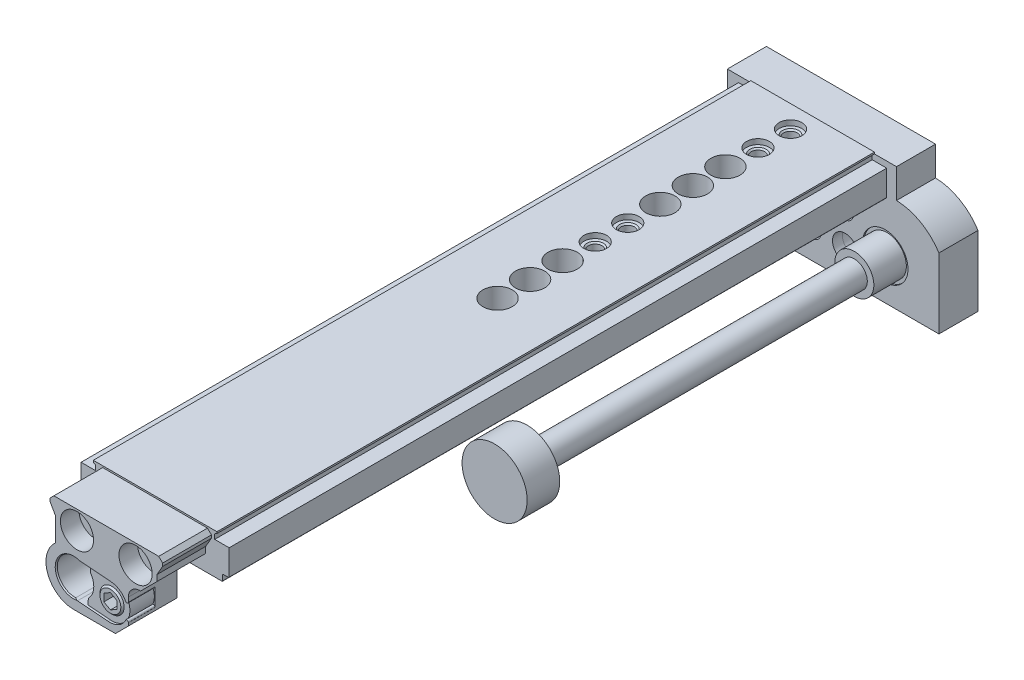
from build123d import *

# Parameters (mm, degrees)
BOSS_EXTRUDE1_DEPTH = 12
CUT_EXTRUDE1_DEPTH  = 3.5
CUT_EXTRUDE2_DEPTH  = 3.5
CUT_EXTRUDE3_DEPTH  = 2.5
SKETCH15_W          = 7
SKETCH15_H          = 0.5
BOSS_EXTRUDE2_DEPTH = 202
BOSS_EXTRUDE3_DEPTH = 15
SKETCH19_R          = 5.1
CUT_EXTRUDE4_DEPTH  = 5.7
SKETCH20_R          = 5.1
CUT_EXTRUDE5_DEPTH  = 5.7
SKETCH21_R          = 2.75
CUT_EXTRUDE6_DEPTH  = 20.6
SKETCH22_R          = 2.75
CUT_EXTRUDE7_DEPTH  = 20.6
SKETCH25_W          = 4.5
SKETCH25_H          = 12.4
SKETCH26_W          = 4.5
SKETCH26_H          = 12.4
SKETCH27_W          = 4.5
SKETCH27_H          = 12.4
SKETCH30_W          = 4.5
SKETCH30_H          = 12.4
SKETCH31_W          = 4.5
SKETCH31_H          = 12.4
SKETCH32_W          = 4.5
SKETCH32_H          = 12.4
CUT_EXTRUDE8_DEPTH  = 8.2
BOSS_EXTRUDE4_START = 7.5
BOSS_EXTRUDE4_DEPTH = 7.5
CUT_EXTRUDE9_DEPTH  = 5.2


with BuildPart() as part:
    # Sketch1 → Boss-Extrude1 (new body)
    with BuildSketch(Plane.XY):
        with BuildLine():
            Line((0, 38), (0, 0))
            Line((0, 0), (65, 0))
            Line((65, 0), (65, 21.556260866))
            ThreePointArc((65, 21.556260866), (59.406255266, 26.898722152), (51.96, 28.992798379))
            Line((51.96, 28.992798379), (51.96, 38))
            Line((51.96, 38), (0, 38))
        make_face()
    extrude(amount=BOSS_EXTRUDE1_DEPTH)

    # Sketch2 → Cut-Revolve1 (revolve, cut)
    with BuildSketch(Plane(origin=(0, 8.5, 0), x_dir=(1, 0, 0), z_dir=(0, 1, 0)), mode=Mode.PRIVATE) as cut_revolve1_sk:
        Polygon((16.2, 0), (20.2, 0), (20.2, -9), (20.1, -9), (20.1, -12), (16.2, -12), align=None)
    revolve(cut_revolve1_sk.sketch.rotate(Axis((16.2, 8.5, 12), (0, 0, -1)), 180), axis=Axis((16.2, 8.5, 12), (0, 0, -1)), mode=Mode.SUBTRACT)

    # Sketch3 → Cut-Revolve2 (revolve, cut)
    with BuildSketch(Plane(origin=(0, 8.5, 0), x_dir=(1, 0, 0), z_dir=(0, 1, 0)), mode=Mode.PRIVATE) as cut_revolve2_sk:
        Polygon((36.2, 0), (40.2, 0), (40.2, -9), (40.1, -9), (40.1, -12), (36.2, -12), align=None)
    revolve(cut_revolve2_sk.sketch.rotate(Axis((36.2, 8.5, 12), (0, 0, -1)), 180), axis=Axis((36.2, 8.5, 12), (0, 0, -1)), mode=Mode.SUBTRACT)

    # Sketch4 → Cut-Revolve3 (revolve, cut)
    with BuildSketch(Plane(origin=(0, 8.5, 0), x_dir=(1, 0, 0), z_dir=(0, 1, 0)), mode=Mode.PRIVATE) as cut_revolve3_sk:
        Polygon((26.2, 0), (29.7, 0), (29.7, -1.6), (28.7, -1.6), (28.267, -1.849992667), (28.267, -11.750007333), (28.7, -12), (26.2, -12), align=None)
    revolve(cut_revolve3_sk.sketch.rotate(Axis((26.2, 8.5, 12), (0, 0, -1)), 180), axis=Axis((26.2, 8.5, 12), (0, 0, -1)), mode=Mode.SUBTRACT)

    # Sketch5 → Cut-Revolve4 (revolve, cut)
    with BuildSketch(Plane(origin=(0, 18.5, 0), x_dir=(1, 0, 0), z_dir=(0, 1, 0)), mode=Mode.PRIVATE) as cut_revolve4_sk:
        Polygon((16.2, 0), (19.7, 0), (19.7, -1.6), (18.7, -1.6), (18.267, -1.849992667), (18.267, -11.750007333), (18.7, -12), (16.2, -12), align=None)
    revolve(cut_revolve4_sk.sketch.rotate(Axis((16.2, 18.5, 12), (0, 0, -1)), 180), axis=Axis((16.2, 18.5, 12), (0, 0, -1)), mode=Mode.SUBTRACT)

    # Sketch6 → Cut-Revolve5 (revolve, cut)
    with BuildSketch(Plane(origin=(0, 18.5, 0), x_dir=(1, 0, 0), z_dir=(0, 1, 0)), mode=Mode.PRIVATE) as cut_revolve5_sk:
        Polygon((26.2, 0), (29.7, 0), (29.7, -1.6), (28.7, -1.6), (28.267, -1.849992667), (28.267, -11.750007333), (28.7, -12), (26.2, -12), align=None)
    revolve(cut_revolve5_sk.sketch.rotate(Axis((26.2, 18.5, 12), (0, 0, -1)), 180), axis=Axis((26.2, 18.5, 12), (0, 0, -1)), mode=Mode.SUBTRACT)

    # Sketch7 → Cut-Revolve6 (revolve, cut)
    with BuildSketch(Plane(origin=(0, 18.5, 0), x_dir=(1, 0, 0), z_dir=(0, 1, 0)), mode=Mode.PRIVATE) as cut_revolve6_sk:
        Polygon((36.2, 0), (39.7, 0), (39.7, -1.6), (38.7, -1.6), (38.267, -1.849992667), (38.267, -11.750007333), (38.7, -12), (36.2, -12), align=None)
    revolve(cut_revolve6_sk.sketch.rotate(Axis((36.2, 18.5, 12), (0, 0, -1)), 180), axis=Axis((36.2, 18.5, 12), (0, 0, -1)), mode=Mode.SUBTRACT)

    # Sketch8 → Cut-Revolve7 (revolve, cut)
    with BuildSketch(Plane(origin=(0, 28.5, 0), x_dir=(1, 0, 0), z_dir=(0, 1, 0)), mode=Mode.PRIVATE) as cut_revolve7_sk:
        Polygon((26.2, 0), (29.7, 0), (29.7, -1.6), (28.7, -1.6), (28.267, -1.849992667), (28.267, -11.750007333), (28.7, -12), (26.2, -12), align=None)
    revolve(cut_revolve7_sk.sketch.rotate(Axis((26.2, 28.5, 12), (0, 0, -1)), 180), axis=Axis((26.2, 28.5, 12), (0, 0, -1)), mode=Mode.SUBTRACT)

    # Sketch9 → Cut-Revolve8 (revolve, cut)
    with BuildSketch(Plane(origin=(0, 32.3, 0), x_dir=(1, 0, 0), z_dir=(0, 1, 0)), mode=Mode.PRIVATE) as cut_revolve8_sk:
        with BuildLine():
            Line((17.2, 0), (22.2, 0))
            Line((22.2, 0), (22.2, -5.7))
            Line((22.2, -5.7), (21.95, -5.7))
            Line((21.95, -5.7), (21.95, -1.1))
            ThreePointArc((21.95, -1.1), (21.832842712, -0.817157288), (21.55, -0.7))
            Line((21.55, -0.7), (19.51, -0.7))
            Line((19.51, -0.7), (17.2, -1.540771241))
            Line((17.2, -1.540771241), (17.2, 0))
        make_face()
    revolve(cut_revolve8_sk.sketch.rotate(Axis((17.2, 32.3, 5.7), (0, 0, -1)), 180), axis=Axis((17.2, 32.3, 5.7), (0, 0, -1)), mode=Mode.SUBTRACT)

    # Sketch10 → Cut-Revolve9 (revolve, cut)
    with BuildSketch(Plane(origin=(0, 32.3, 0), x_dir=(1, 0, 0), z_dir=(0, 1, 0)), mode=Mode.PRIVATE) as cut_revolve9_sk:
        with BuildLine():
            Line((35.2, 0), (40.2, 0))
            Line((40.2, 0), (40.2, -5.7))
            Line((40.2, -5.7), (39.95, -5.7))
            Line((39.95, -5.7), (39.95, -1.1))
            ThreePointArc((39.95, -1.1), (39.832842712, -0.817157288), (39.55, -0.7))
            Line((39.55, -0.7), (37.51, -0.7))
            Line((37.51, -0.7), (35.2, -1.540771241))
            Line((35.2, -1.540771241), (35.2, 0))
        make_face()
    revolve(cut_revolve9_sk.sketch.rotate(Axis((35.2, 32.3, 5.7), (0, 0, -1)), 180), axis=Axis((35.2, 32.3, 5.7), (0, 0, -1)), mode=Mode.SUBTRACT)

    # Sketch11 → Cut-Extrude1 (cut)
    with BuildSketch(Plane(origin=(0, 0, 0.7), x_dir=(-1, 0, 0), z_dir=(0, 0, -1))):
        Polygon((-33.2, 33.454700538), (-35.2, 34.609401077), (-37.2, 33.454700538), (-37.2, 31.145299462), (-35.2, 29.990598923), (-33.2, 31.145299462), align=None)
    extrude(amount=-CUT_EXTRUDE1_DEPTH, mode=Mode.SUBTRACT)

    # Sketch12 → Cut-Extrude2 (cut)
    with BuildSketch(Plane(origin=(0, 0, 0.7), x_dir=(-1, 0, 0), z_dir=(0, 0, -1))):
        Polygon((-15.2, 33.454700538), (-17.2, 34.609401077), (-19.2, 33.454700538), (-19.2, 31.145299462), (-17.2, 29.990598923), (-15.2, 31.145299462), align=None)
    extrude(amount=-CUT_EXTRUDE2_DEPTH, mode=Mode.SUBTRACT)

    # Sketch13 → Cut-Revolve10 (revolve, cut)
    with BuildSketch(Plane(origin=(0, 12.5, 0), x_dir=(1, 0, 0), z_dir=(0, 1, 0)), mode=Mode.PRIVATE) as cut_revolve10_sk:
        with BuildLine():
            Line((48.5, 0), (53.5, 0))
            Line((53.5, 0), (53.5, -5.7))
            Line((53.5, -5.7), (52.75, -5.7))
            Line((52.75, -5.7), (52.75, -1.1))
            ThreePointArc((52.75, -1.1), (52.632842712, -0.817157288), (52.35, -0.7))
            Line((52.35, -0.7), (50.81, -0.7))
            Line((50.81, -0.7), (48.5, -1.540771241))
            Line((48.5, -1.540771241), (48.5, 0))
        make_face()
    revolve(cut_revolve10_sk.sketch.rotate(Axis((48.5, 12.5, 5.7), (0, 0, -1)), 180), axis=Axis((48.5, 12.5, 5.7), (0, 0, -1)), mode=Mode.SUBTRACT)

    # Sketch14 → Cut-Extrude3 (cut)
    with BuildSketch(Plane(origin=(0, 0, 0.7), x_dir=(-1, 0, 0), z_dir=(0, 0, -1))):
        Polygon((-46.5, 13.654700538), (-48.5, 14.809401077), (-50.5, 13.654700538), (-50.5, 11.345299462), (-48.5, 10.190598923), (-46.5, 11.345299462), align=None)
    extrude(amount=-CUT_EXTRUDE3_DEPTH, mode=Mode.SUBTRACT)

    # Sketch15 → Cut-Revolve11 (revolve, cut)
    with BuildSketch(Plane(origin=(0, 12.5, 0), x_dir=(1, 0, 0), z_dir=(0, 1, 0)), mode=Mode.PRIVATE) as cut_revolve11_sk:
        with Locations((52, -11.75)):
            Rectangle(SKETCH15_W, SKETCH15_H)
    revolve(cut_revolve11_sk.sketch.rotate(Axis((48.5, 12.5, 12), (0, 0, -1)), 180), axis=Axis((48.5, 12.5, 12), (0, 0, -1)), mode=Mode.SUBTRACT)

    # Sketch16 → Revolve1 (revolve)
    with BuildSketch(Plane(origin=(0, 12.5, 0), x_dir=(1, 0, 0), z_dir=(0, 1, 0)), mode=Mode.PRIVATE) as revolve1_sk:
        Polygon((48.5, -11.5), (54.5, -11.5), (54.5, -21.5), (52.5, -21.5), (52.5, -122), (58.5, -122), (58.5, -132), (48.5, -132), align=None)
    revolve(revolve1_sk.sketch.rotate(Axis((48.5, 12.5, 132), (0, 0, -1)), 180), axis=Axis((48.5, 12.5, 132), (0, 0, -1)))

    # Sketch17 → Boss-Extrude2 (add)
    with BuildSketch(Plane.XY.offset(12)):
        with BuildLine():
            Line((3.45, 36.1), (3.45, 28.05))
            ThreePointArc((3.45, 28.05), (3.508578644, 27.908578644), (3.65, 27.85))
            Line((3.65, 27.85), (5.25, 27.85))
            ThreePointArc((5.25, 27.85), (5.391421356, 27.791421356), (5.45, 27.65))
            Line((5.45, 27.65), (5.45, 26.3))
            ThreePointArc((5.45, 26.3), (5.508578644, 26.158578644), (5.65, 26.1))
            Line((5.65, 26.1), (46.75, 26.1))
            ThreePointArc((46.75, 26.1), (46.891421356, 26.158578644), (46.95, 26.3))
            Line((46.95, 26.3), (46.95, 27.9))
            ThreePointArc((46.95, 27.9), (47.008578644, 28.041421356), (47.15, 28.1))
            Line((47.15, 28.1), (48.75, 28.1))
            ThreePointArc((48.75, 28.1), (48.891421356, 28.158578644), (48.95, 28.3))
            Line((48.95, 28.3), (48.95, 36.1))
            Line((48.95, 36.1), (44.5, 36.1))
            Line((44.5, 36.1), (44.5, 37.595854812))
            Line((44.5, 37.595854812), (45.2, 38))
            Line((45.2, 38), (45.2, 38.5))
            Line((45.2, 38.5), (7.2, 38.5))
            Line((7.2, 38.5), (7.2, 38))
            Line((7.2, 38), (7.9, 37.595854812))
            Line((7.9, 37.595854812), (7.9, 36.1))
            Line((7.9, 36.1), (3.45, 36.1))
        make_face()
    extrude(amount=BOSS_EXTRUDE2_DEPTH)

    # Sketch18 → Boss-Extrude3 (add)
    with BuildSketch(Plane.XY.offset(214)):
        with BuildLine():
            Line((16.18, 10.8), (29, 10.8))
            Line((29, 10.8), (33, 14.8))
            Line((33, 14.8), (33, 22.5))
            ThreePointArc((33, 22.5), (34.025126266, 24.974873734), (36.5, 26))
            Line((36.5, 26), (36.75, 26))
            Line((36.75, 26), (41.75, 31))
            Line((41.75, 31), (41.75, 32.868911087))
            Line((41.75, 32.868911087), (43.5, 35.9))
            Line((43.5, 35.9), (43.5, 36.8))
            Line((43.5, 36.8), (42.3, 38))
            Line((42.3, 38), (10.1, 38))
            Line((10.1, 38), (8.9, 36.8))
            Line((8.9, 36.8), (8.9, 35.9))
            Line((8.9, 35.9), (10.65, 32.868911087))
            Line((10.65, 32.868911087), (10.65, 25.755160726))
            ThreePointArc((10.65, 25.755160726), (8.207582983, 16.352023251), (16.18, 10.8))
        make_face()
    extrude(amount=BOSS_EXTRUDE3_DEPTH)

    # Sketch19 → Cut-Extrude4 (cut)
    with BuildSketch(Plane.XY.offset(229)):
        with Locations((17.2, 32.3)):
            Circle(SKETCH19_R)
    extrude(amount=-CUT_EXTRUDE4_DEPTH, mode=Mode.SUBTRACT)

    # Sketch20 → Cut-Extrude5 (cut)
    with BuildSketch(Plane.XY.offset(229)):
        with Locations((35.2, 32.3)):
            Circle(SKETCH20_R)
    extrude(amount=-CUT_EXTRUDE5_DEPTH, mode=Mode.SUBTRACT)

    # Sketch21 → Cut-Extrude6 (cut)
    with BuildSketch(Plane.XY.offset(229)):
        with Locations((17.2, 32.3)):
            Circle(SKETCH21_R)
    extrude(amount=-CUT_EXTRUDE6_DEPTH, mode=Mode.SUBTRACT)

    # Sketch22 → Cut-Extrude7 (cut)
    with BuildSketch(Plane.XY.offset(229)):
        with Locations((35.2, 32.3)):
            Circle(SKETCH22_R)
    extrude(amount=-CUT_EXTRUDE7_DEPTH, mode=Mode.SUBTRACT)

    # Sketch23 → Cut-Revolve12 (revolve, cut)
    with BuildSketch(Plane(origin=(26.2, 0, 0), x_dir=(0, 0, -1), z_dir=(1, 0, 0)), mode=Mode.PRIVATE) as cut_revolve12_sk:
        Polygon((-18.8, 38.5), (-15.3, 38.5), (-15.3, 36.9), (-16.3, 36.9), (-16.733, 36.467), (-16.733, 26.533), (-16.3, 26.1), (-18.8, 26.1), align=None)
    revolve(cut_revolve12_sk.sketch.rotate(Axis((26.2, 26.1, 18.8), (0, 1, 0)), 180), axis=Axis((26.2, 26.1, 18.8), (0, 1, 0)), mode=Mode.SUBTRACT)

    # Sketch24 → Cut-Revolve13 (revolve, cut)
    with BuildSketch(Plane(origin=(26.2, 0, 0), x_dir=(0, 0, -1), z_dir=(1, 0, 0)), mode=Mode.PRIVATE) as cut_revolve13_sk:
        Polygon((-28.8, 38.5), (-25.3, 38.5), (-25.3, 36.9), (-26.3, 36.9), (-26.733, 36.467), (-26.733, 26.533), (-26.3, 26.1), (-28.8, 26.1), align=None)
    revolve(cut_revolve13_sk.sketch.rotate(Axis((26.2, 26.1, 28.8), (0, 1, 0)), 180), axis=Axis((26.2, 26.1, 28.8), (0, 1, 0)), mode=Mode.SUBTRACT)

    # Sketch25 → Cut-Revolve14 (revolve, cut)
    with BuildSketch(Plane(origin=(26.2, 0, 0), x_dir=(0, 0, -1), z_dir=(1, 0, 0)), mode=Mode.PRIVATE) as cut_revolve14_sk:
        with Locations((-36.55, 32.3)):
            Rectangle(SKETCH25_W, SKETCH25_H)
    revolve(cut_revolve14_sk.sketch.rotate(Axis((26.2, 26.1, 38.8), (0, 1, 0)), 180), axis=Axis((26.2, 26.1, 38.8), (0, 1, 0)), mode=Mode.SUBTRACT)

    # Sketch26 → Cut-Revolve15 (revolve, cut)
    with BuildSketch(Plane(origin=(26.2, 0, 0), x_dir=(0, 0, -1), z_dir=(1, 0, 0)), mode=Mode.PRIVATE) as cut_revolve15_sk:
        with Locations((-46.55, 32.3)):
            Rectangle(SKETCH26_W, SKETCH26_H)
    revolve(cut_revolve15_sk.sketch.rotate(Axis((26.2, 26.1, 48.8), (0, 1, 0)), 180), axis=Axis((26.2, 26.1, 48.8), (0, 1, 0)), mode=Mode.SUBTRACT)

    # Sketch27 → Cut-Revolve16 (revolve, cut)
    with BuildSketch(Plane(origin=(26.2, 0, 0), x_dir=(0, 0, -1), z_dir=(1, 0, 0)), mode=Mode.PRIVATE) as cut_revolve16_sk:
        with Locations((-56.55, 32.3)):
            Rectangle(SKETCH27_W, SKETCH27_H)
    revolve(cut_revolve16_sk.sketch.rotate(Axis((26.2, 26.1, 58.8), (0, 1, 0)), 180), axis=Axis((26.2, 26.1, 58.8), (0, 1, 0)), mode=Mode.SUBTRACT)

    # Sketch28 → Cut-Revolve17 (revolve, cut)
    with BuildSketch(Plane(origin=(26.2, 0, 0), x_dir=(0, 0, -1), z_dir=(1, 0, 0)), mode=Mode.PRIVATE) as cut_revolve17_sk:
        Polygon((-68.8, 38.5), (-65.3, 38.5), (-65.3, 36.9), (-66.3, 36.9), (-66.733, 36.467), (-66.733, 26.533), (-66.3, 26.1), (-68.8, 26.1), align=None)
    revolve(cut_revolve17_sk.sketch.rotate(Axis((26.2, 26.1, 68.8), (0, 1, 0)), 180), axis=Axis((26.2, 26.1, 68.8), (0, 1, 0)), mode=Mode.SUBTRACT)

    # Sketch29 → Cut-Revolve18 (revolve, cut)
    with BuildSketch(Plane(origin=(26.2, 0, 0), x_dir=(0, 0, -1), z_dir=(1, 0, 0)), mode=Mode.PRIVATE) as cut_revolve18_sk:
        Polygon((-78.8, 38.5), (-75.3, 38.5), (-75.3, 36.9), (-76.3, 36.9), (-76.733, 36.467), (-76.733, 26.533), (-76.3, 26.1), (-78.8, 26.1), align=None)
    revolve(cut_revolve18_sk.sketch.rotate(Axis((26.2, 26.1, 78.8), (0, 1, 0)), 180), axis=Axis((26.2, 26.1, 78.8), (0, 1, 0)), mode=Mode.SUBTRACT)

    # Sketch30 → Cut-Revolve19 (revolve, cut)
    with BuildSketch(Plane(origin=(26.2, 0, 0), x_dir=(0, 0, -1), z_dir=(1, 0, 0)), mode=Mode.PRIVATE) as cut_revolve19_sk:
        with Locations((-86.55, 32.3)):
            Rectangle(SKETCH30_W, SKETCH30_H)
    revolve(cut_revolve19_sk.sketch.rotate(Axis((26.2, 26.1, 88.8), (0, 1, 0)), 180), axis=Axis((26.2, 26.1, 88.8), (0, 1, 0)), mode=Mode.SUBTRACT)

    # Sketch31 → Cut-Revolve20 (revolve, cut)
    with BuildSketch(Plane(origin=(26.2, 0, 0), x_dir=(0, 0, -1), z_dir=(1, 0, 0)), mode=Mode.PRIVATE) as cut_revolve20_sk:
        with Locations((-96.55, 32.3)):
            Rectangle(SKETCH31_W, SKETCH31_H)
    revolve(cut_revolve20_sk.sketch.rotate(Axis((26.2, 26.1, 98.8), (0, 1, 0)), 180), axis=Axis((26.2, 26.1, 98.8), (0, 1, 0)), mode=Mode.SUBTRACT)

    # Sketch32 → Cut-Revolve21 (revolve, cut)
    with BuildSketch(Plane(origin=(26.2, 0, 0), x_dir=(0, 0, -1), z_dir=(1, 0, 0)), mode=Mode.PRIVATE) as cut_revolve21_sk:
        with Locations((-106.55, 32.3)):
            Rectangle(SKETCH32_W, SKETCH32_H)
    revolve(cut_revolve21_sk.sketch.rotate(Axis((26.2, 26.1, 108.8), (0, 1, 0)), 180), axis=Axis((26.2, 26.1, 108.8), (0, 1, 0)), mode=Mode.SUBTRACT)

    # Sketch33 → Cut-Extrude8 (cut)
    with BuildSketch(Plane.XY.offset(229)):
        with BuildLine():
            Line((17.363542707, 13.691420111), (26.834257378, 12.946058702))
            ThreePointArc((26.834257378, 12.946058702), (30.051430893, 13.686724624), (32.264961371, 16.136025395))
            ThreePointArc((32.264961371, 16.136025395), (32.741551731, 16.099832892), (32.97, 15.68))
            Line((32.97, 15.68), (33.95, 15.68))
            Line((33.95, 15.68), (33.95, 21.18))
            Line((33.95, 21.18), (32.97, 21.18))
            ThreePointArc((32.97, 21.18), (32.741073917, 20.759858439), (32.263924274, 20.724442325))
            ThreePointArc((32.263924274, 20.724442325), (30.413907196, 22.939016486), (27.697307431, 23.912149373))
            Line((27.697307431, 23.912149373), (18.22659276, 24.657510782))
            ThreePointArc((18.22659276, 24.657510782), (12.312022398, 19.605990473), (17.363542707, 13.691420111))
        make_face()
    extrude(amount=-CUT_EXTRUDE8_DEPTH, mode=Mode.SUBTRACT)

    # Sketch34 → Boss-Extrude4 (add)
    with BuildSketch(Plane.XY.offset(220.8).offset(BOSS_EXTRUDE4_START)):
        with BuildLine():
            Line((19.855836042, 13.495272372), (26.834257378, 12.946058702))
            ThreePointArc((26.834257378, 12.946058702), (32.74882774, 17.997579011), (27.697307431, 23.912149373))
            Line((27.697307431, 23.912149373), (20.718886095, 24.461363043))
            Line((20.718886095, 24.461363043), (19.855836042, 13.495272372))
        make_face()
    extrude(amount=-BOSS_EXTRUDE4_DEPTH)

    # Sketch35 → Cut-Revolve22 (revolve, cut)
    with BuildSketch(Plane(origin=(16.2, 0, 0), x_dir=(0, 0, -1), z_dir=(1, 0, 0)), mode=Mode.PRIVATE) as cut_revolve22_sk:
        Polygon((-229, 19.3), (-229, 24.989440108), (-228.6, 24.7585), (-214.4, 24.7585), (-214, 24.989440108), (-214, 19.3), align=None)
    revolve(cut_revolve22_sk.sketch.rotate(Axis((16.2, 19.3, 214), (0, 0, 1)), 270), axis=Axis((16.2, 19.3, 214), (0, 0, 1)), mode=Mode.SUBTRACT)

    # Sketch36 → Revolve2 (revolve)
    with BuildSketch(Plane(origin=(27.265782404, 0, 0), x_dir=(0, 0, -1), z_dir=(1, 0, 0)), mode=Mode.PRIVATE) as revolve2_sk:
        Polygon((-220.8, 18.429104037), (-220.8, 14.429104037), (-228, 14.429104037), (-228.8, 15.229104037), (-228.8, 18.429104037), align=None)
    revolve(revolve2_sk.sketch.rotate(Axis((27.265782404, 18.429104037, 228.8), (0, 0, -1)), 90), axis=Axis((27.265782404, 18.429104037, 228.8), (0, 0, -1)))

    # Sketch37 → Cut-Extrude9 (cut)
    with BuildSketch(Plane.XY.offset(229)):
        Polygon((25.265782404, 17.274403499), (27.265782404, 16.119702961), (29.265782404, 17.274403499), (29.265782404, 19.583804576), (27.265782404, 20.738505114), (25.265782404, 19.583804576), align=None)
    extrude(amount=-CUT_EXTRUDE9_DEPTH, mode=Mode.SUBTRACT)


solid = part.part
